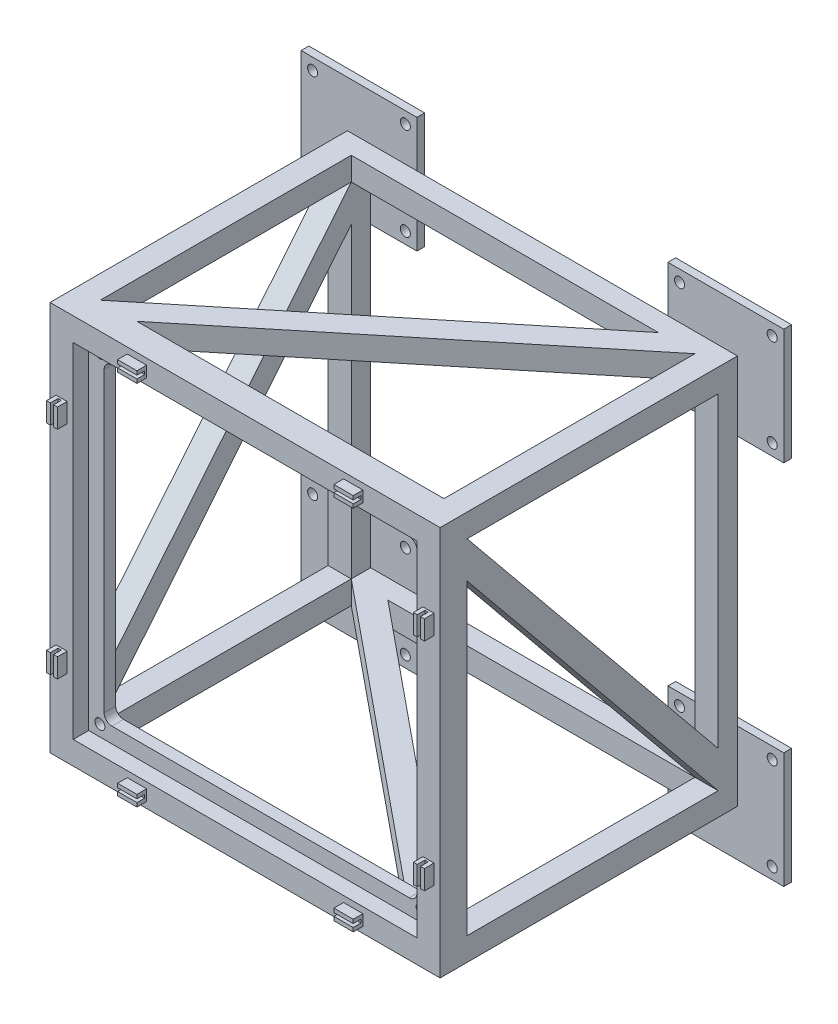
from build123d import *

# Parameters (mm, degrees)
SKETCH1_W           = 1010
SKETCH1_H           = 1010
BOSS_EXTRUDE1_DEPTH = 770
SKETCH2_W           = 890
SKETCH2_H           = 650
CUT_EXTRUDE1_DEPTH  = 445
CUT_EXTRUDE2_DEPTH  = 60
CIRPATTERN2_COUNT   = 4
SKETCH5_W           = 890
SKETCH5_H           = 890
CUT_EXTRUDE3_DEPTH  = 1065
SKETCH6_W           = 890
SKETCH6_H           = 890
SKETCH6_W_2         = 810
SKETCH6_H_2         = 810
BOSS_EXTRUDE2_DEPTH = 30
FILLET1_R           = 20
SKETCH7_R           = 13
CUT_EXTRUDE4_DEPTH  = 30
SKETCH8_W           = 300
SKETCH8_H           = 300
SKETCH8_R           = 13
BOSS_EXTRUDE3_DEPTH = 20
CIRPATTERN3_COUNT   = 4
SKETCH9_W           = 50
SKETCH9_H           = 28.5
SKETCH9_W_2         = 28.5
SKETCH9_H_2         = 50
BOSS_EXTRUDE4_DEPTH = 25
SKETCH10_W          = 1191.407960266
SKETCH10_H          = 8.5
CUT_EXTRUDE5_DEPTH  = 20
CIRPATTERN4_COUNT   = 4


with BuildPart() as part:
    # Sketch1 → Boss-Extrude1 (new body)
    with BuildSketch(Plane.XY):
        Rectangle(SKETCH1_W, SKETCH1_H)
    extrude(amount=BOSS_EXTRUDE1_DEPTH)

    # Sketch2 → Cut-Extrude1 (cut, symmetric)
    with BuildSketch(Plane(origin=(0, 0, 0), x_dir=(1, 0, 0), z_dir=(0, 1, 0))):
        with Locations((0, -375)):
            Rectangle(SKETCH2_W, SKETCH2_H)
    extrude(amount=CUT_EXTRUDE1_DEPTH, both=True, mode=Mode.SUBTRACT)

    # Sketch3 → Cut-Extrude2 (cut)
    with BuildSketch(Plane.ZY.offset(505)):
        Polygon((700, -350.195216969), (700, 445), (50, 445), align=None)
        Polygon((50, 350.195216969), (50, -445), (700, -445), align=None)
    cut_extrude2 = extrude(amount=-CUT_EXTRUDE2_DEPTH, mode=Mode.SUBTRACT)

    # CirPattern2: Cut-Extrude2 ×4 about axis
    cirpattern2_axis = Axis((0, 0, 0), (0, 0, 1))
    for i in range(1, CIRPATTERN2_COUNT):
        add(cut_extrude2.rotate(cirpattern2_axis, i * 360 / CIRPATTERN2_COUNT), mode=Mode.SUBTRACT)

    # Sketch5 → Cut-Extrude3 (cut)
    with BuildSketch(Plane.XY.offset(770)):
        Rectangle(SKETCH5_W, SKETCH5_H)
    extrude(amount=-CUT_EXTRUDE3_DEPTH, mode=Mode.SUBTRACT)

    # Sketch6 → Boss-Extrude2 (add)
    with BuildSketch(Plane(origin=(0, 0, 700), x_dir=(-1, 0, 0), z_dir=(0, 0, -1))):
        Rectangle(SKETCH6_W, SKETCH6_H)
        Rectangle(SKETCH6_W_2, SKETCH6_H_2, mode=Mode.SUBTRACT)
    extrude(amount=-BOSS_EXTRUDE2_DEPTH)

    # Fillet1
    fillet1_edges = [part.edges().sort_by_distance(p)[0] for p in [
        (405, 405, 715),
        (-405, 405, 715),
        (-405, -405, 715),
        (405, -405, 715),
    ]]
    fillet(fillet1_edges, radius=FILLET1_R)

    # Sketch7 → Cut-Extrude4 (cut)
    with BuildSketch(Plane.XY.offset(730)):
        with Locations((-416, 416)):
            Circle(SKETCH7_R)
        with Locations((416, 416)):
            Circle(SKETCH7_R)
        with Locations((416, -416)):
            Circle(SKETCH7_R)
        with Locations((-416, -416)):
            Circle(SKETCH7_R)
    extrude(amount=-CUT_EXTRUDE4_DEPTH, mode=Mode.SUBTRACT)

    # Sketch8 → Boss-Extrude3 (add)
    with BuildSketch(Plane(origin=(0, 0, 0), x_dir=(-1, 0, 0), z_dir=(0, 0, -1))):
        with Locations((-475, -475)):
            Rectangle(SKETCH8_W, SKETCH8_H)
        with Locations((-595, -355)):
            Circle(SKETCH8_R, mode=Mode.SUBTRACT)
        with Locations((-355, -355)):
            Circle(SKETCH8_R, mode=Mode.SUBTRACT)
        with Locations((-595, -595)):
            Circle(SKETCH8_R, mode=Mode.SUBTRACT)
        with Locations((-355, -595)):
            Circle(SKETCH8_R, mode=Mode.SUBTRACT)
    boss_extrude3 = extrude(amount=BOSS_EXTRUDE3_DEPTH)

    # CirPattern3: Boss-Extrude3 ×4 about axis
    cirpattern3_axis = Axis((0, 0, 0), (0, 0, 1))
    for i in range(1, CIRPATTERN3_COUNT):
        add(boss_extrude3.rotate(cirpattern3_axis, i * 360 / CIRPATTERN3_COUNT))

    # Sketch9 → Boss-Extrude4 (add)
    with BuildSketch(Plane.XY.offset(770)):
        with Locations((-280, -475)):
            Rectangle(SKETCH9_W, SKETCH9_H)
        with Locations((280, -475)):
            Rectangle(SKETCH9_W, SKETCH9_H)
        with Locations((-475, 280)):
            Rectangle(SKETCH9_W_2, SKETCH9_H_2)
        with Locations((-475, -280)):
            Rectangle(SKETCH9_W_2, SKETCH9_H_2)
        with Locations((280, 475)):
            Rectangle(SKETCH9_W, SKETCH9_H)
        with Locations((-280, 475)):
            Rectangle(SKETCH9_W, SKETCH9_H)
        with Locations((475, -280)):
            Rectangle(SKETCH9_W_2, SKETCH9_H_2)
        with Locations((475, 280)):
            Rectangle(SKETCH9_W_2, SKETCH9_H_2)
    extrude(amount=BOSS_EXTRUDE4_DEPTH)

    # Sketch10 → Cut-Extrude5 (cut)
    with BuildSketch(Plane.XY.offset(795)):
        with Locations((-255, -475)):
            Rectangle(SKETCH10_W, SKETCH10_H)
    cut_extrude5 = extrude(amount=-CUT_EXTRUDE5_DEPTH, mode=Mode.SUBTRACT)

    # CirPattern4: Cut-Extrude5 ×4 about axis
    cirpattern4_axis = Axis((0, 0, 0), (0, 0, 1))
    for i in range(1, CIRPATTERN4_COUNT):
        add(cut_extrude5.rotate(cirpattern4_axis, i * 360 / CIRPATTERN4_COUNT), mode=Mode.SUBTRACT)


solid = part.part
